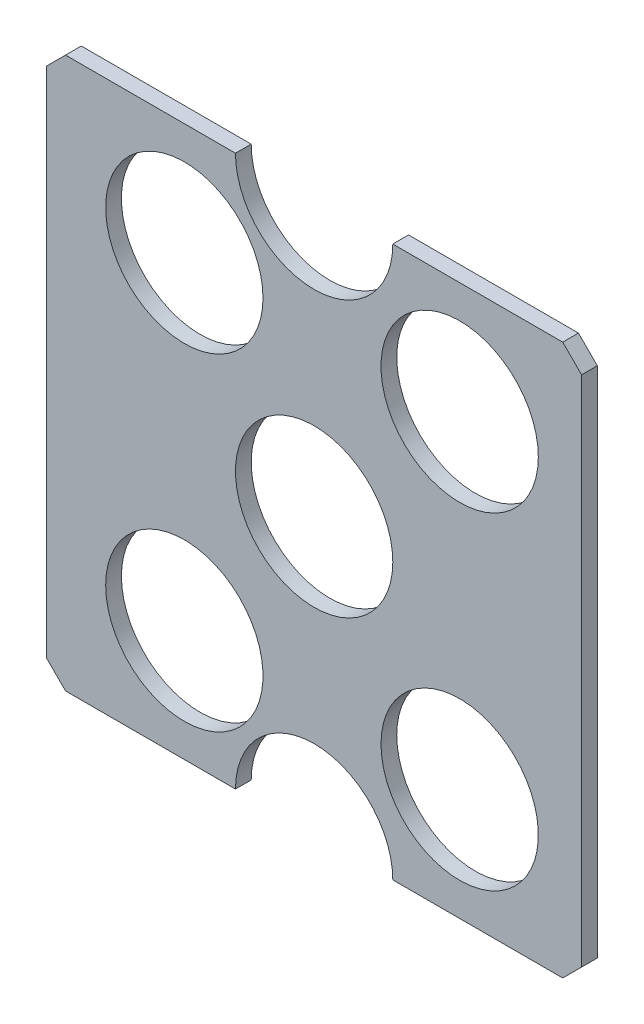
SolidWorks part; units mm, degrees
ref_plane "Front Plane" through (0, 0, 0) normal (0, 0, 1) x (1, 0, 0)
ref_plane "Top Plane" through (0, 0, 0) normal (0, 1, 0) x (1, 0, 0)
ref_plane "Right Plane" through (0, 0, 0) normal (1, 0, 0) x (0, 0, -1)
sketch "Sketch1" plane through (0, 0, 0) normal (0, 0, 1) x (1, 0, 0)
  line L0 (0, 175) -> (378.4163, 175) construction
  line L1 (12, 0) -> (120, 0)
  line L2 (0, 12) -> (0, 338)
  line L3 (12, 350) -> (120, 350)
  line L4 (340, 12) -> (340, 338)
  line L5 (170, 350) -> (170, -15.8441) construction
  line L6 (220, 350) -> (328, 350)
  line L7 (220, 0) -> (328, 0)
  line L8 (0, 338) -> (12, 350)
  line L9 (0, 12) -> (12, 0)
  line L10 (328, 0) -> (340, 12)
  line L11 (340, 338) -> (328, 350)
  arc A0 (220, 0) -> (120, 0) centre (170, 0) ccw
  arc A1 (120, 350) -> (220, 350) centre (170, 350) ccw
  circle A2 centre (170, 175) radius 50
  circle A3 centre (87.5, 279) radius 50
  circle A4 centre (262.5, 279) radius 50
  circle A5 centre (87.5, 71) radius 50
  circle A6 centre (262.5, 71) radius 50
  point P0 (0, 0)
  point P1 (340, 350)
  point P2 (0, 350)
  point P3 (340, 0)
  dimension "D3" = 100
  dimension "D4" = 100
  dimension "D5" = 100
  dimension "D6" = 100
  dimension "D7" = 100
  dimension "D1" = 350
  dimension "D2" = 340
  dimension "D8" = 87.5
  dimension "D9" = 175
  dimension "D10" = 104
  dimension "D11" = 104
  dimension "D12" = 12
  dimension "D13" = 45
  dimension "D14" = 12
  dimension "D15" = 45
  dimension "D16" = 12
  dimension "D17" = 45
  dimension "D18" = 12
  dimension "D19" = 45
extrude "Boss-Extrude1" add sketch "Sketch1" along normal blind 10
